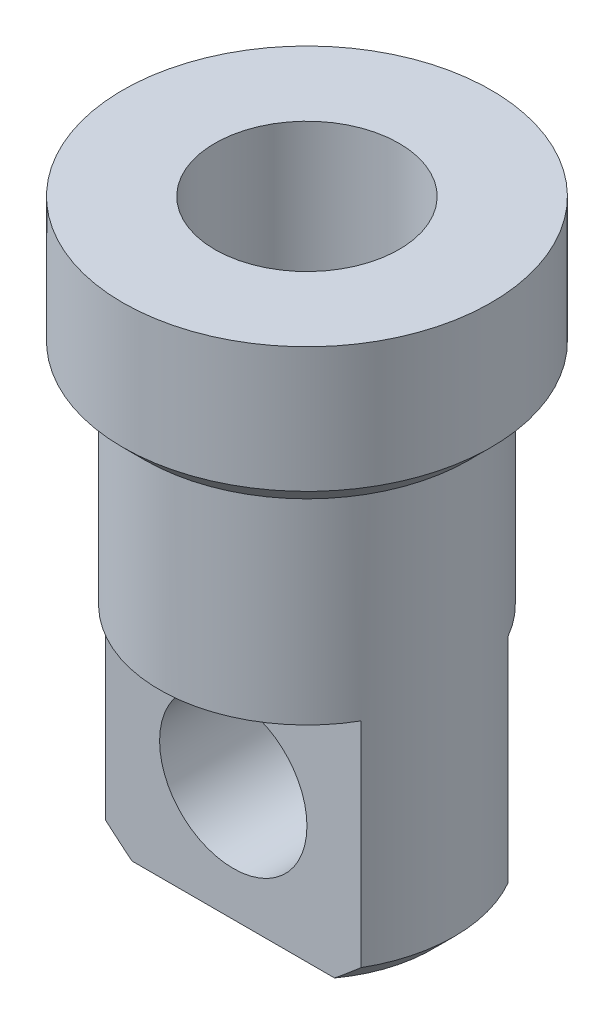
SolidWorks part; units mm, degrees
ref_plane "Front Plane" through (0, 0, 0) normal (0, 0, 1) x (1, 0, 0)
ref_plane "Top Plane" through (0, 0, 0) normal (0, 1, 0) x (1, 0, 0)
ref_plane "Right Plane" through (0, 0, 0) normal (1, 0, 0) x (0, 0, -1)
sketch "Sketch1" plane through (0, 0, 0) normal (0, 1, 0) x (1, 0, 0)
  circle A0 centre (0, 0) radius 2
  dimension "D1" = 4
extrude "Boss-Extrude1" add sketch "Sketch1" along normal blind 6
sketch "Sketch2" plane through (0, 6, 0) normal (0, 1, 0) x (1, 0, 0)
  circle A0 centre (0, 0) radius 2.5
  dimension "D1" = 5
extrude "Boss-Extrude2" add sketch "Sketch2" along normal blind 2
hole_wizard "M3 Tapped Hole1" positions "Sketch5" profile "Sketch4" tap size "M3" standard "Gb"
sketch "Sketch5" plane through (0, 8, 0) normal (0, 1, 0) x (1, 0, 0)
  point P0 (0, 0)
sketch "Sketch4" plane through (0, 8, 0) normal (1, 0, 0) x (0, 0, 1)
  line L0 (0, 0) -> (0, 5.2511)
  line L1 (0, 5.2511) -> (1.25, 4.5)
  line L2 (1.25, 4.5) -> (1.25, 0)
  line L5 (1.25, 0) -> (0, 0)
  line L10 (0, 5.2511) -> (-1.25, 4.5) construction
  line L11 (0, -6.35) -> (0, 107.95) construction
  dimension "螺纹孔钻头直径" = 2.5
  dimension "螺纹孔钻头深度" = 4.5
  dimension "导头角度" = 118
cosmetic thread "Cosmetic Thread1" parameters "D1"=4.5, "D2"=3
chamfer "Chamfer1" distance 0.3 angle 45 2 edges at (0, 0, 2) (0, 6, 2.5)
sketch "Sketch6" plane through (0, 0, 0) normal (0, 0, 1) x (1, 0, 0)
  line L0 (0, 0) -> (0, 50000) construction
  line L1 (-1.7, 0) -> (1.7, 0) construction
  circle A0 centre (0, 1.6) radius 1
  dimension "D1" = 2
  dimension "D2" = 1.6
extrude "Cut-Extrude1" cut sketch "Sketch6" against normal mid plane 10
sketch "Sketch7" plane through (0, 0, 0) normal (1, 0, 0) x (0, 0, -1)
  line L0 (0, 0) -> (0, 50000) construction
  line L1 (-0.488, 1.6) -> (49999.512, 1.6) construction
  line L2 (-1.7, 0) -> (1.7, 0) construction
  line L3 (4, 0) -> (1, 0)
  line L4 (4, 0) -> (4, 3.2)
  line L5 (4, 3.2) -> (1, 3.2)
  line L6 (1, 0) -> (1, 3.2)
  line L7 (4, 0) -> (1, 3.2) construction
  line L8 (4, 3.2) -> (1, 0) construction
  line L9 (-4, 3.2) -> (-1, 0) construction
  line L10 (-4, 0) -> (-1, 3.2) construction
  line L11 (1.7521, 1.6) -> (-49998.2479, 1.6) construction
  line L12 (-1, 0) -> (-1, 3.2)
  line L13 (-4, 3.2) -> (-1, 3.2)
  line L14 (-4, 0) -> (-4, 3.2)
  line L15 (-4, 0) -> (-1, 0)
  point P5 (2.5, 1.6)
  point P18 (-2.5, 1.6)
  dimension "D1" = 1.6
  dimension "D2" = 2
  dimension "D3" = 3.2
  dimension "D4" = 8
extrude "Cut-Extrude2" cut sketch "Sketch7" against normal mid plane 10
